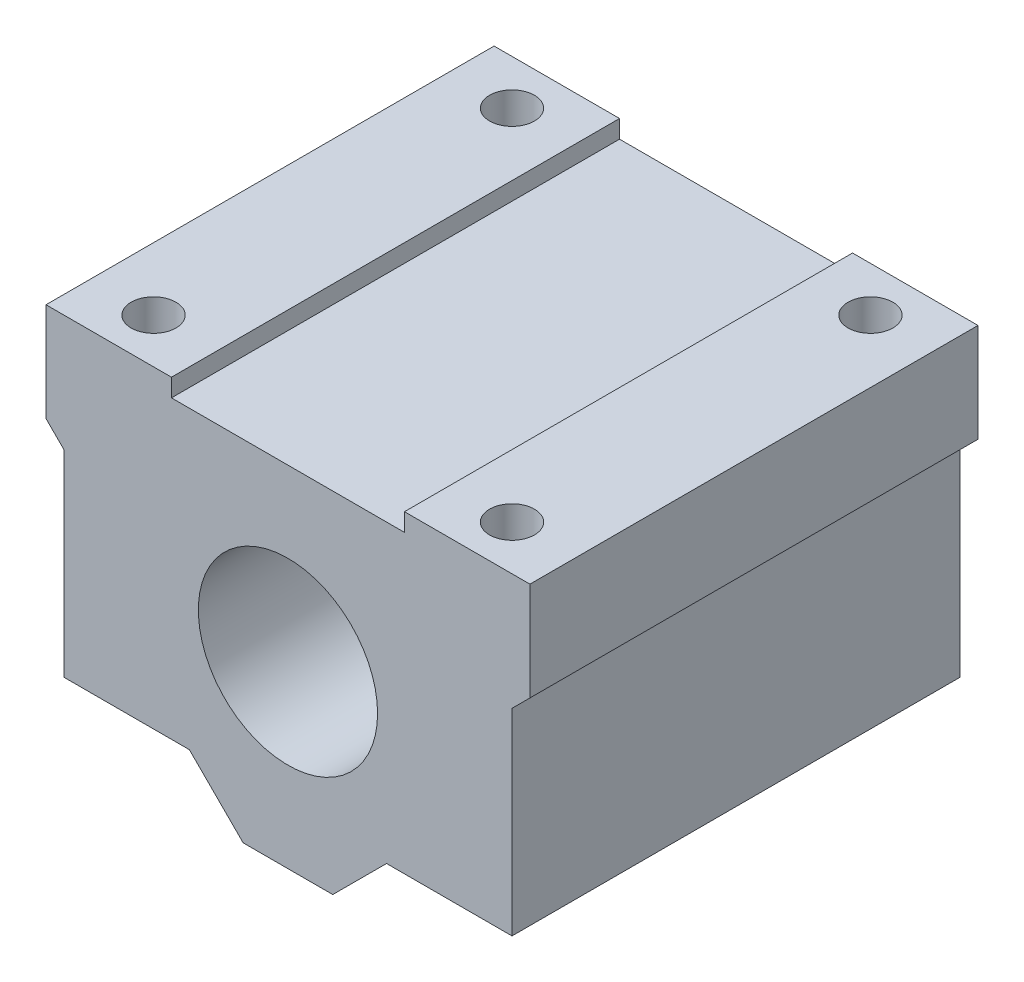
from build123d import *

# Parameters (mm, degrees)
SKETCH_1_R                  = 10
EXTRUDE_1_DEPTH             = 50
PATTERN_LINEAR_1_COUNT      = 2
PATTERN_LINEAR_1_PITCH      = 40
PATTERN_LINEAR_1_COUNT_DIR2 = 2
PATTERN_LINEAR_1_PITCH_DIR2 = 40


with BuildPart() as part:
    # 草图1 → 拉伸1 (new body)
    with BuildSketch(Plane.XY):
        Polygon((5, -20), (-5, -20), (-11, -14), (-25, -14), (-25, 8), (-27, 10), (-27, 21), (-13, 21), (-13, 19), (13, 19), (13, 21), (27, 21), (27, 10), (25, 8), (25, -14), (11, -14), align=None)
        Circle(SKETCH_1_R, mode=Mode.SUBTRACT)
    extrude(amount=EXTRUDE_1_DEPTH)

    # 草图2 → M6x1.0 螺纹孔1 (revolve, cut)
    with BuildSketch(Plane(origin=(20, 21, 5), x_dir=(0, 0, 1), z_dir=(1, 0, 0))):
        Polygon((0, 0), (0, 18.502151548), (2.5, 17), (2.5, 0), align=None)
    m6x1_0_1 = revolve(axis=Axis((20, 27.35, 5), (0, -1, 0)), mode=Mode.SUBTRACT)

    # 阵列(线性)1: M6x1.0 _1 2 × 2
    with Locations(*[(-j * PATTERN_LINEAR_1_PITCH_DIR2, 0, i * PATTERN_LINEAR_1_PITCH) for i in range(PATTERN_LINEAR_1_COUNT) for j in range(PATTERN_LINEAR_1_COUNT_DIR2) if (i, j) != (0, 0)]):
        add(m6x1_0_1, mode=Mode.SUBTRACT)


solid = part.part
